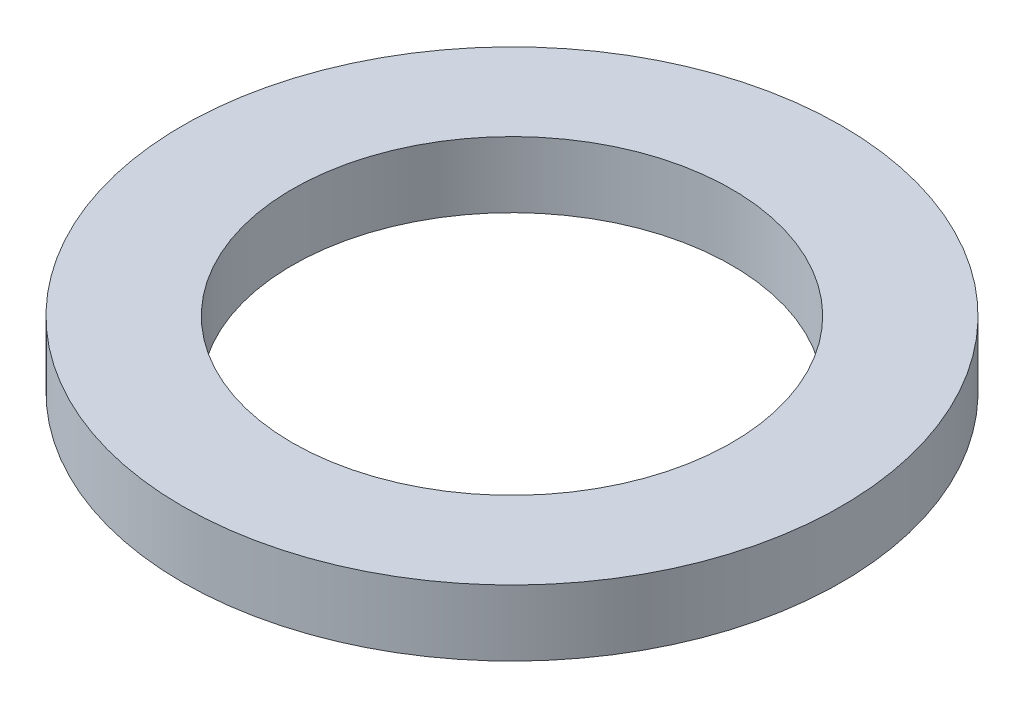
SolidWorks part; units mm, degrees
ref_plane "Front Plane" through (0, 0, 0) normal (0, 0, 1) x (1, 0, 0)
ref_plane "Top Plane" through (0, 0, 0) normal (0, 1, 0) x (1, 0, 0)
ref_plane "Right Plane" through (0, 0, 0) normal (1, 0, 0) x (0, 0, -1)
sketch "Sketch1" plane through (0, 0, 0) normal (0, 1, 0) x (1, 0, 0)
  circle A0 centre (0, 0) radius 15
  circle A1 centre (0, 0) radius 10
extrude "Boss-Extrude1" add sketch "Sketch1" along normal blind 3
ref_plane "Plane1" through (0, 0, 15) normal (0, 0, 1) x (1, 0, 0)
sketch "Sketch2" plane through (0, 0, 15) normal (0, 0, 1) x (1, 0, 0)
  circle A0 centre (0, 1.5) radius 1.5
